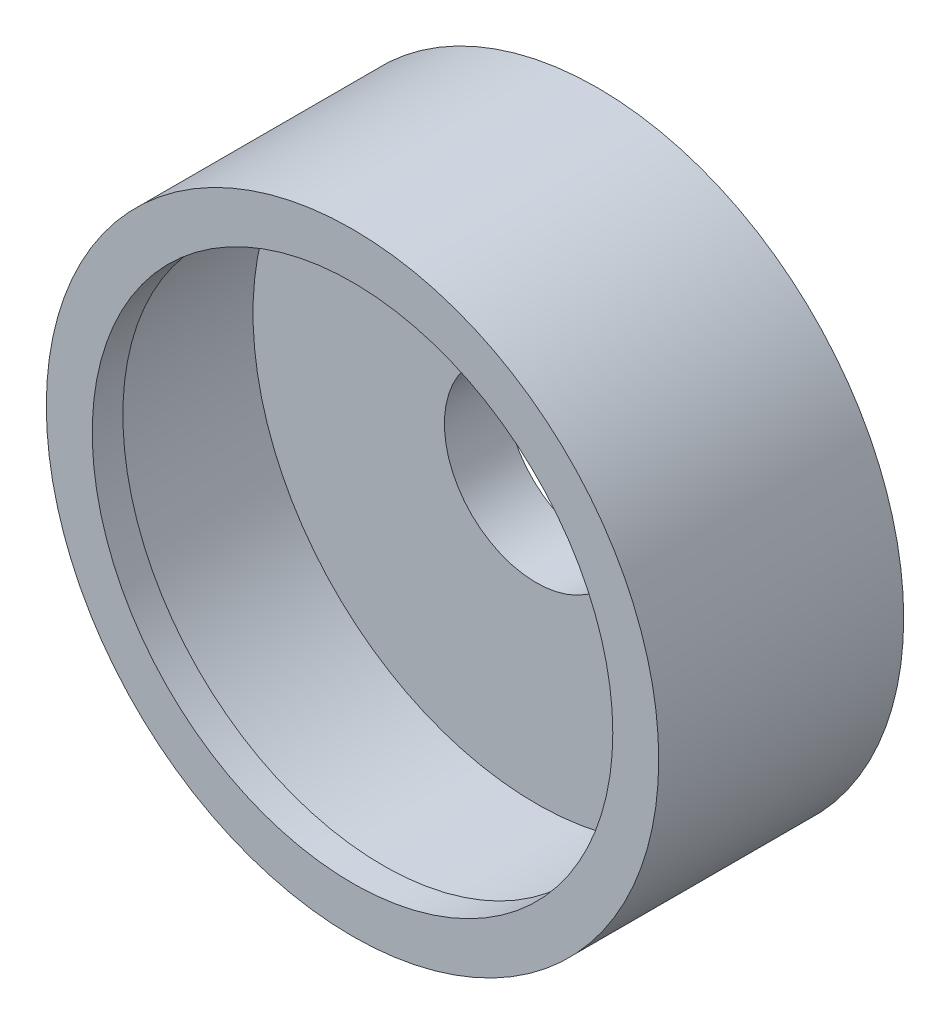
SolidWorks part; units mm, degrees
material "SUS304"
ref_plane "Front Plane" through (0, 0, 0) normal (0, 0, 1) x (1, 0, 0)
ref_plane "Top Plane" through (0, 0, 0) normal (0, 1, 0) x (1, 0, 0)
ref_plane "Right Plane" through (0, 0, 0) normal (1, 0, 0) x (0, 0, -1)
sketch "Sketch1" plane through (0, 0, 0) normal (0, 0, 1) x (1, 0, 0)
  circle A0 centre (0, 0) radius 10
  dimension "D1" = 20
extrude "Boss-Extrude1" add sketch "Sketch1" along normal blind 8
sketch "Sketch2" plane through (0, 0, 8) normal (0, 0, 1) x (1, 0, 0)
  circle A0 centre (0, 0) radius 8.5
  dimension "D1" = 17
extrude "Cut-Extrude1" cut sketch "Sketch2" against normal blind 6
sketch "Sketch3" plane through (0, 0, 2) normal (0, 0, 1) x (1, 0, 0)
  circle A0 centre (0, 0) radius 3
  dimension "D1" = 6
extrude "Cut-Extrude2" cut sketch "Sketch3" against normal through all
sketch "Sketch4" plane through (0, 0, 2) normal (0, 0, 1) x (1, 0, 0)
  circle A0 centre (0, 0) radius 9.25
  dimension "D1" = 18.5
extrude "Cut-Extrude3" cut sketch "Sketch4" along normal blind 5
